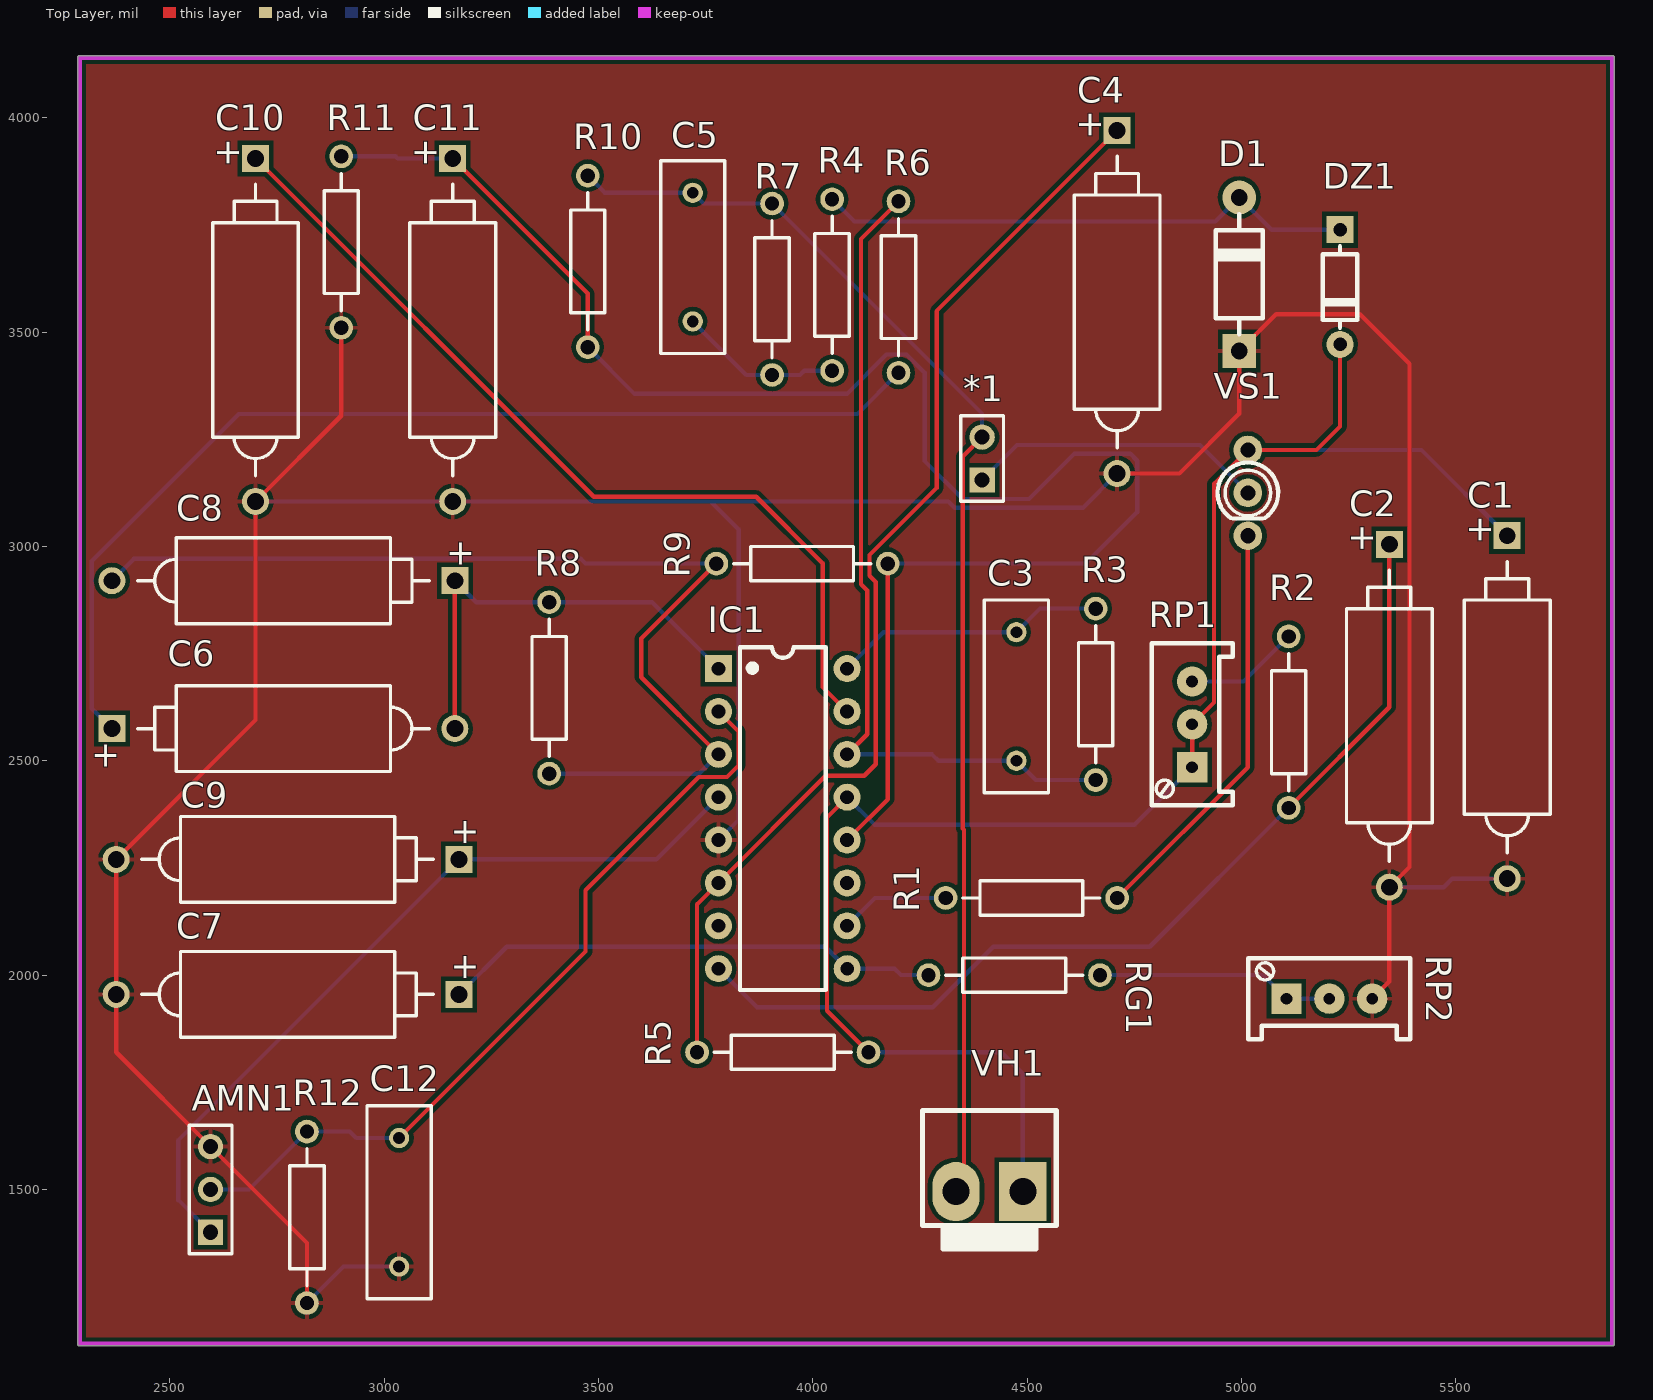
[diagram p0: Top Layer view]
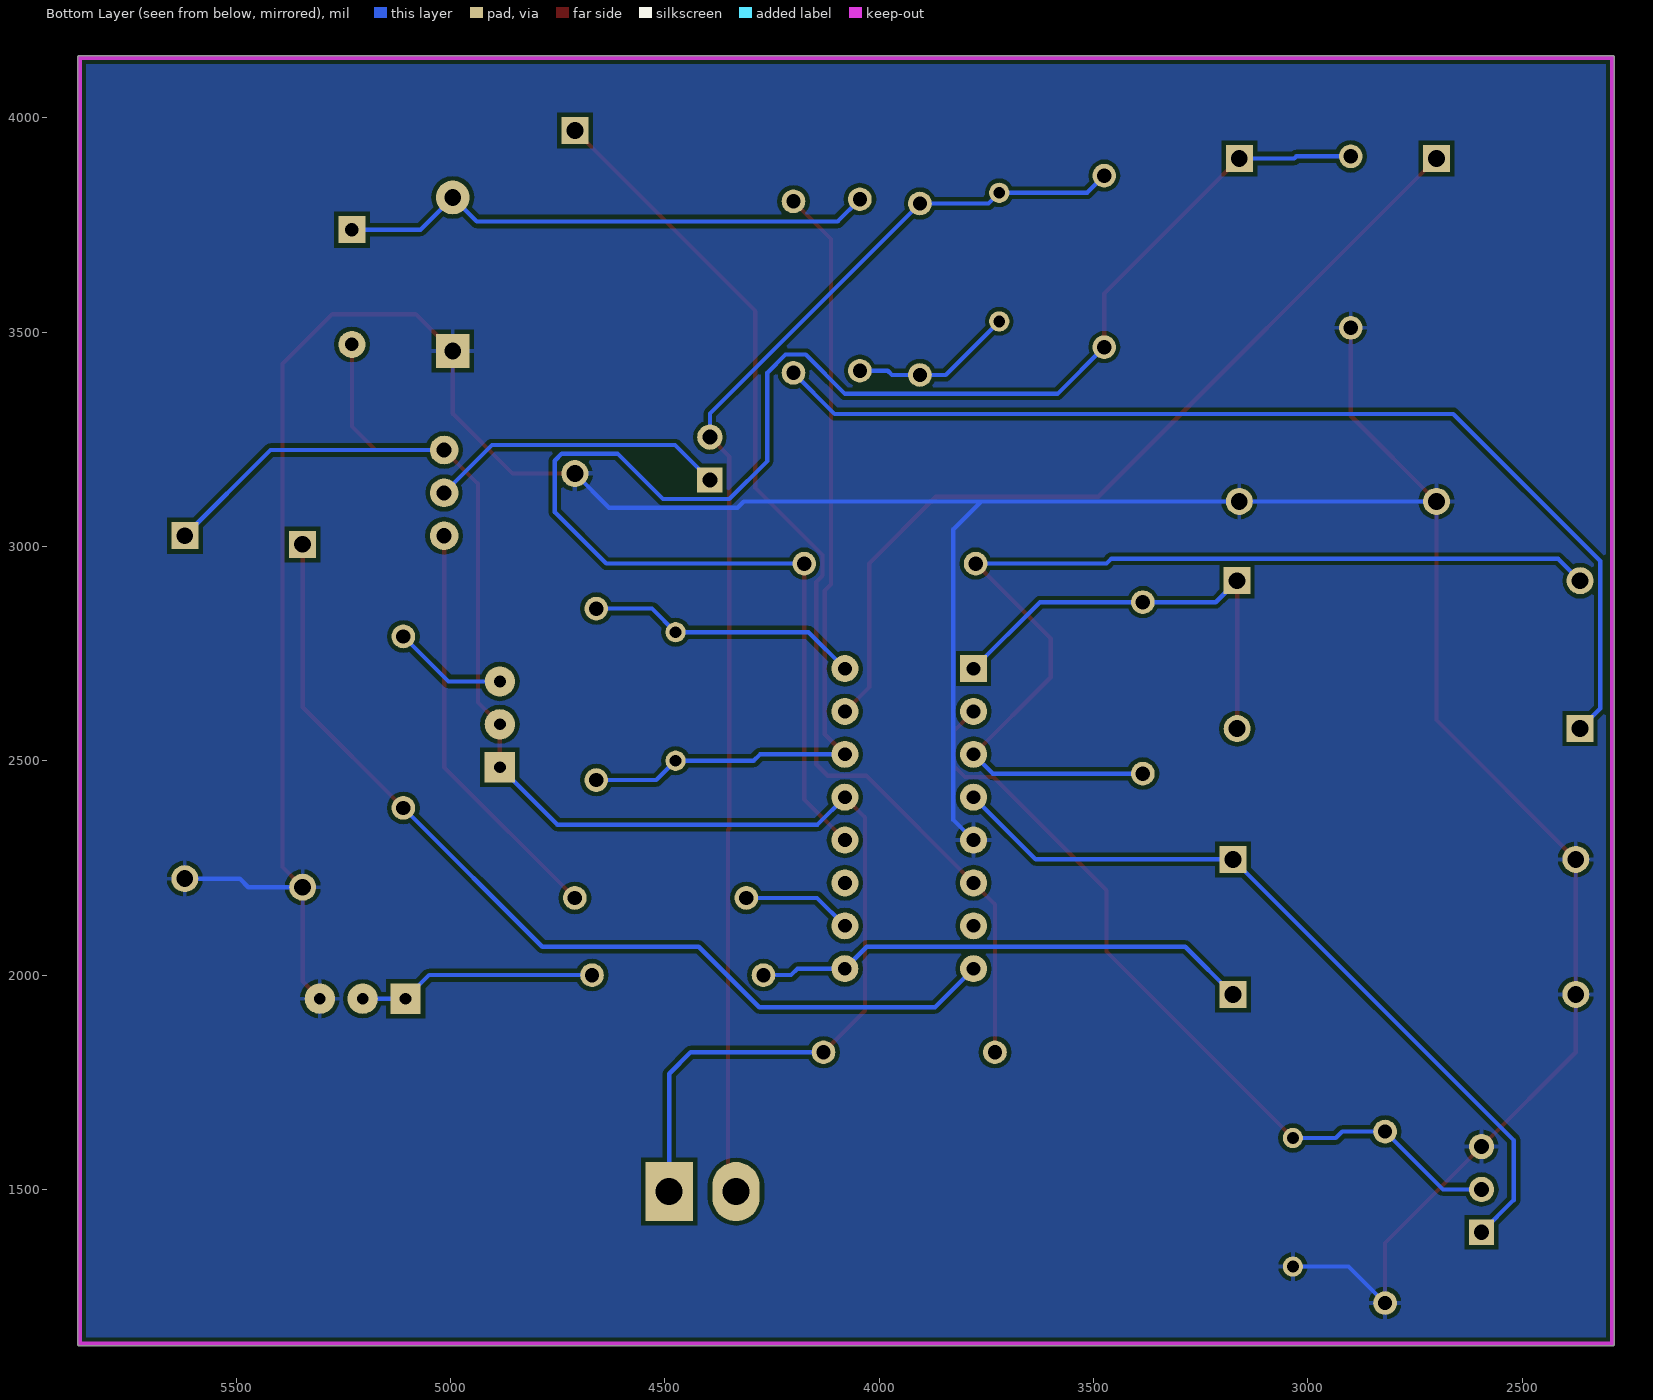
[diagram p1: Bottom Layer view, seen from below]
# Altium PCB MISC82068.PcbDoc
Units mil, origin at the board's own origin, x right, y up, seen from the top; angles counter-clockwise.
Board outline 3585.03 x 3010.03 mil, 2 copper layers (Top Layer, Bottom Layer); 34 components, 22 nets, 86 pads, 0 vias.

## Layer stack, top to bottom (the 12.6 mil dielectric is the usual default, probably not edited)
Top Solder: solder mask 0.4, Solder Resist, Dk 3.5
Top Layer: signal copper 1.4
Dielectric 1: dielectric 12.6, FR-4, Dk 4.8
Bottom Layer: signal copper 1.4
Bottom Solder: solder mask 0.4, Solder Resist, Dk 3.5

## Board outline
2284.99,1140 ccw(c2290,1140) 2290,1134.98 5865,1134.98 ccw(c5865,1140) 5870.02,1140 5870.02,4140 ccw(c5865,4140) 5865,4145.02 2290,4145.02 ccw(c2290,4140) 2284.99,4140

## Design rules (kind name [scope] priority, off if disabled: settings)
Clearance [All] p1: gap=10
PolygonConnect [All] p1: connectstyle=Relief reliefconductorwidth=10 reliefentries=4 polygonreliefangle="90 Angle" airgapwidth=10
RoutingVias [All] p1: holewidth=28 width=50 viastyle="Through Hole" minholewidth=28 minwidth=50 maxholewidth=28 maxwidth=50
SolderMaskExpansion [All] p1: expansion=4
Width [All] p1: maxlimit=10 minlimit=10 preferedwidth=10
30 further rules are at their usual default settings.

## Components (designator, comment, footprint, x,y, rotation, side; value= is the part's Value field where it differs from the comment)
*1 "H" HDR1X2 4395,3155 r90 top
AMN1 "PIR" HDR1X3 2595,1400 r90 top
C1 "470U" POLAR0.8 5620,2625 r90 top
C2 "100U" POLAR0.8 5345,2605 r90 top
C3 "0.047U" RAD-0.3 4475,2650 r90 top
C4 "4.7U" POLAR0.8 4710,3570 r90 top
C5 "0.1U" RAD-0.3 3720,3675 r270 top
C6 "47U" POLAR0.8 2765,2575 r180 top
C7 "4.7U" POLAR0.8 2775,1955 r0 top
C8 "1U" POLAR0.8 2765,2920 r0 top
C9 "100U" POLAR0.8 2775,2270 r0 top
C10 "22U" POLAR0.8 2700,3505 r90 top
C11 "33U" POLAR0.8 3160,3505 r90 top
C12 "0.01U" RAD-0.3 3035,1470 r90 top
D1 "1N4007" DO-41 4995,3635 r90 top
DZ1 "5.1V" DO-35 5230,3605 r270 top
IC1 "TDH98072" DIP16 3780,2715 r0 top
R1 "330K" AXIAL-0.4 4510,2180 r180 top
R2 "4.7K" AXIAL-0.4 5110,2590 r270 top
R3 "500K" AXIAL-0.4 4660,2655 r90 top
R4 "47" AXIAL-0.4 4045,3610 r90 top
R5 "100K" AXIAL-0.4 3930,1820 r180 top
R6 "15K" AXIAL-0.4 4200,3605 r90 top
R7 "100K" AXIAL-0.4 3905,3600 r270 top
R8 "320K" AXIAL-0.4 3385,2670 r90 top
R9 "15K" AXIAL-0.4 3975,2960 r180 top
R10 "1M" AXIAL-0.4 3475,3665 r90 top
R11 "470K" AXIAL-0.4 2900,3710 r90 top
R12 "47K" AXIAL-0.4 2820,1435 r90 top
RG1 "10K" AXIAL-0.4 4470,2000 r0 top
RP1 "1M" 3296W 4885,2585 r90 top
RP2 "1M" 3296W 5205,1945 r0 top
VH1 "220V" VH3.96-2A 4490,1495 r180 top
VS1 "1A/600V" "LED 3mm-2P" 5015,3125 r270 top

## Footprints (in the part's own frame and the unit in brackets; to place one, negate y for a bottom-side part, rotate by r counter-clockwise, add the part's x,y. Pads: shape width x height; smd on the part's side, far side on the other; paste and mask are expansions set on the pad)
3296W [mm] "Precise Multi-Winding Adjustable Resistor"
  rect 1.8x1.8 hole 0.7: 1(-2.54,0)
  round 1.8 hole 0.7: 2(0,0) 3(2.54,0)
  silkscreen extent -4.8,-2.4 4.8,2.4, body extent -4.75,-2.4 4.75,2.4, height 11.52
AXIAL-0.4 [mm] "Axial Device, Thru-Hole; 2 Leads; 0.4 in Pin Spacing"
  round 1.4 hole 0.85: 1(-5.08,0) 2(5.08,0)
  silkscreen extent -4.06,-1.02 4.06,1.02
DIP16 [mm]
  rect 1.6x1.6 hole 0.813: 1(0,0)
  round 1.6 hole 0.813: 2(0,-2.54) 3(0,-5.08) 4(0,-7.62) 5(0,-10.16) 6(0,-12.7) 7(0,-15.24) 8(0,-17.78) 9(7.627,-17.78) 10(7.62,-15.24) 11(7.62,-12.7) 12(7.62,-10.16) 13(7.62,-7.62) 14(7.62,-5.08) 15(7.62,-2.54) 16(7.62,0)
  silkscreen extent 1.27,-19.05 6.35,1.27, body extent -0.12,-18.76 7.75,1.24, height 5.1
DO-35 [mm] "1.8*6.8mm(直径，脚距）"
  rect 1.6x1.6 hole 0.8: 1(-3.4,0)
  round 1.6 hole 0.8: 2(3.4,0)
  silkscreen extent -2.41,-1.02 2.41,1.02, body extent -3.65,-0.9 3.65,0.9, height 1.85
DO-41 [mm] "2.6*9.1mm(直径，脚距）"
  rect 2x2 hole 1: 1(-4.55,0)
  round 2 hole 1: 2(4.55,0)
  silkscreen extent -3.56,-1.4 3.56,1.4, body extent -4.92,-1.29 4.98,1.31, height 2.65
HDR1X2 [mm] "Connector; Header; 2 Position"
  rect 1.5x1.5 hole 0.9: 1(0,0)
  round 1.5 hole 0.9: 2(2.54,0)
  silkscreen extent -1.27,-1.27 3.81,1.27
HDR1X3 [mm] "Connector; Header; 3 Position"
  rect 1.5x1.5 hole 0.9: 1(0,0)
  round 1.5 hole 0.9: 2(2.54,0) 3(5.08,0)
  silkscreen extent -1.27,-1.27 6.35,1.27
"LED 3mm-2P" [mm] "3mm˫ɫLED"
  round 1.7 hole 0.9: 1(0,0) 2(-2.54,0) 3(2.54,0)
  silkscreen extent -1.8,-1.79 1.52,1.79, body extent -2.79,-1.95 2.79,1.95, height 6.9
POLAR0.8 [mm] "Polarized Capacitor; 2 Leads"
  rect 1.6x1.6 hole 1: 1(10.16,0)
  round 1.6 hole 1: 2(-10.16,0)
  silkscreen extent -8.64,-2.54 8.64,2.54
RAD-0.3 [mm] "Radial Cap, Thru-Hole; 2 Leads; 0.3 in Pin Spacing"
  round 1.2 hole 0.7: 1(-3.81,0) 2(3.81,0)
  silkscreen extent -5.71,-1.91 5.71,1.91
VH3.96-2A [mm]
  rect 2.8x3.5 hole 1.6: 1(0,0)
  oval 2.8x3.5 hole 1.6: 2(3.96,0)
  silkscreen extent -1.98,-4.8 5.94,3.4, body extent -1.98,-4.8 5.94,3.6, height 14.6

## Part data
C1 C2 C4 C6 C7 C8 C9 C10 C11: library part "Cap Pol2", "Polarized Capacitor (Axial)"
C3 C5 C12: library part Cap, "Capacitor"
D1: "Rectifier diode"
DZ1: library part 1N4619, "3V/0.5W Zener diode"
R1 R2 R3 R4 R5 R6 R7 R8 R9 R10 R11 R12: library part Res2, "Resistor"
RG1: library part RG, "Photoresistor"
RP1 RP2: library part RP, "Single potentiometer"
VH1: library part VH2

## Nets (pads, with @x,y where several pads share a name; then routed paths per layer and width w, separated by ;. In a path a pad name is that pad's centre, name@x,y a point inside that pad or via, vN(x,y) a via of type N, cw(c..) or ccw(c..) an arc to the next point about the centre after c; other vN are vias at no path point)
GND: AMN1.3 C1.2 C2.2 C4.2 C7.2 C9.2 C10.2 C11.2 C12.1 D1.1 IC1.5 R11.1 R12.1 RP2.3 | length 8582.3
  Top Layer w10: R12.1 2820,1375 AMN1.3 2375,1820 C7.2 C9.2 2700,2595 C10.2 2900,3305 R11.1 ; C4.2 4855.13,3170 4995,3309.87 D1.1 5081.13,3542 5276,3542 5392,3426 5392,2252 C2.2 5345,1985 RP2.3
  Bottom Layer w10: C10.2 C11.2 3762,3105 ; R12.1 2905,1320 C12.1 ; IC1.5 3827,2362 3827,3040 3762,3105 ; C4.2 4630.47,3090.47 4330.47,3090.47 4315.94,3105 3762,3105 ; C2.2 5472,2205 5492,2225 C1.2
Net*1_1: *1.1 VS1.1 | length 699.9
  Bottom Layer w10: *1.1 4476.5,3236.5 4903.5,3236.5 VS1.1
Net*1_2: *1.2 C5.1 R7.1 R10.2 VH1.2 | length 3003.7
  Top Layer w10: VH1.2 4353,1495 4353,2339 4350,2342 4350,3210 *1.2
  Bottom Layer w10: R10.2 3515,3825 C5.1 3745,3800 R7.1 4395,3310 *1.2
NetAMN1_1: AMN1.1 C9.1 IC1.4 | length 1837.4
  Bottom Layer w10: AMN1.1 2520,1475 2520,1615 C9.1 3635.01,2270 IC1.4
NetAMN1_2: AMN1.2 C12.2 IC1.2 R12.2 | length 1883.3
  Top Layer w10: C12.2 3470,2055 3470,2198 3734,2462 3800,2462 3827,2489 3827,2568 IC1.2
  Bottom Layer w10: AMN1.2 2685,1500 R12.2 2920,1635 2935,1620 C12.2
NetC1_1: C1.1 DZ1.2 IC1.13 R5.1 RP1.1 RP1.2 VH1.1 VS1.2 | length 4108
  Top Layer w10: IC1.13 4033,2368 4033,1917 R5.1 ; RP1.1 RP1.2 4936,2636 4936,3146 VS1.2 5175,3225 5230,3280 DZ1.2
  Bottom Layer w10: IC1.13 4144,2351 4751,2351 RP1.1 ; R5.1 4440,1820 4490,1770 VH1.1 ; VS1.2 5420,3225 C1.1
NetC2_1: C2.1 IC1.8 R2.2 | length 2272.2
  Top Layer w10: R2.2 5345,2625 C2.1
  Bottom Layer w10: IC1.8 3869.99,1925 4280,1925 4421,2066 4786,2066 R2.2
NetC3_1: C3.1 IC1.14 R3.1 R6.2 | length 1956.6
  Top Layer w10: IC1.14 4127,2562 4127,2897.44 4112.44,2912 4112.44,3717.44 R6.2
  Bottom Layer w10: IC1.14 4278,2515 4293,2500 C3.1 4520,2455 R3.1
NetC3_2: C3.2 IC1.16 R3.2 | length 638
  Bottom Layer w10: IC1.16 4165.01,2800 C3.2 4530,2855 R3.2
NetC4_1: C4.1 IC1.6 R5.2 | length 2620.7
  Top Layer w10: R5.2 3730,2165 IC1.6 4030,2465 4120,2465 4147,2492 4147,2917 4132.44,2931.56 4132.44,2980 4289,3136.56 4289,3549 C4.1
NetC5_2: C5.2 R4.1 R7.2 | length 380.9
  Bottom Layer w10: C5.2 3845,3400 R7.2 3970,3400 3980,3410 R4.1
NetC6_1: C6.1 R6.1 | length 2474.3
  Bottom Layer w10: C6.1 2318,2622 2318,2966 2661,3309 4104,3309 R6.1
NetC6_2: C6.2 C8.1 IC1.1 R8.2 | length 1044.9
  Top Layer w10: C6.2 C8.1
  Bottom Layer w10: C8.1 3215,2870 R8.2 3625,2870 IC1.1
NetC7_1: C7.1 IC1.9 RG1.1 | length 1168.3
  Bottom Layer w10: C7.1 3286,2066 4029.28,2066 IC1.9 4190.72,2015 4205.72,2000 RG1.1
NetC8_2: C8.2 IC1.3 R8.1 R9.2 | length 2441.4
  Top Layer w10: R9.2 3600,2785 3600,2695 IC1.3
  Bottom Layer w10: C8.2 2416,2971 3459,2971 3470,2960 R9.2 ; R8.1 3735,2470 IC1.3
NetC10_1: C10.1 IC1.15 | length 2083.6
  Top Layer w10: C10.1 3489,3116 3868,3116 4023,2961 4023,2672 IC1.15
NetC11_1: C11.1 IC1.12 R9.1 R10.1 R11.2 | length 3944.5
  Top Layer w10: C11.1 3475,3590 R10.1 ; IC1.12 4175,2409.99 R9.1
  Bottom Layer w10: R11.2 3027,3910 3032,3905 C11.1 ; R10.1 3584,3356 4080,3356 4171.56,3447.56 4218.44,3447.56 4261,3405 4261,3199.47 4350,3110.47 4504.47,3110.47 4610.5,3216.5 4740.5,3216.5 4757,3200 4757,3080 4637,2960 R9.1
NetD1_2: D1.2 DZ1.1 R4.2 | length 1261
  Bottom Layer w10: R4.2 4097,3758 4938.87,3758 D1.2 5070.28,3738.86 DZ1.1
NetIC1_10: IC1.10 R1.2 | length 256.9
  Bottom Layer w10: IC1.10 4145,2180 R1.2
NetR1_1: R1.1 VS1.3 | length 971.3
  Top Layer w10: R1.1 5015,2485 VS1.3
NetR2_1: R2.1 RP1.3 | length 268.5
  Bottom Layer w10: RP1.3 5005,2685 R2.1
NetRG1_2: RG1.2 RP2.1 RP2.2 | length 557.8
  Bottom Layer w10: RG1.2 5050,2000 RP2.1 RP2.2
pads on no net: IC1.7 IC1.11

## Polygon pours and split planes (outlines as drawn)
GND on Top Layer "D" (solid, remove dead copper, pour order 0): 1950,4360 1995,4405 6720,4405 6720,1720 6090,1090 6015,1015 2075,1015
GND on Bottom Layer "D" (solid, remove dead copper, pour order 2): 1955,4525 6660,4525 6995,4190 6170,3365 6170,1225 6170,865 6110,805 6065,760 2015,760

## Keep-outs
Keep-Out Layer:
  lines w10: 2290,3910 2290,4140 5865,4140 5865,1140 2290,1140 2290,3970